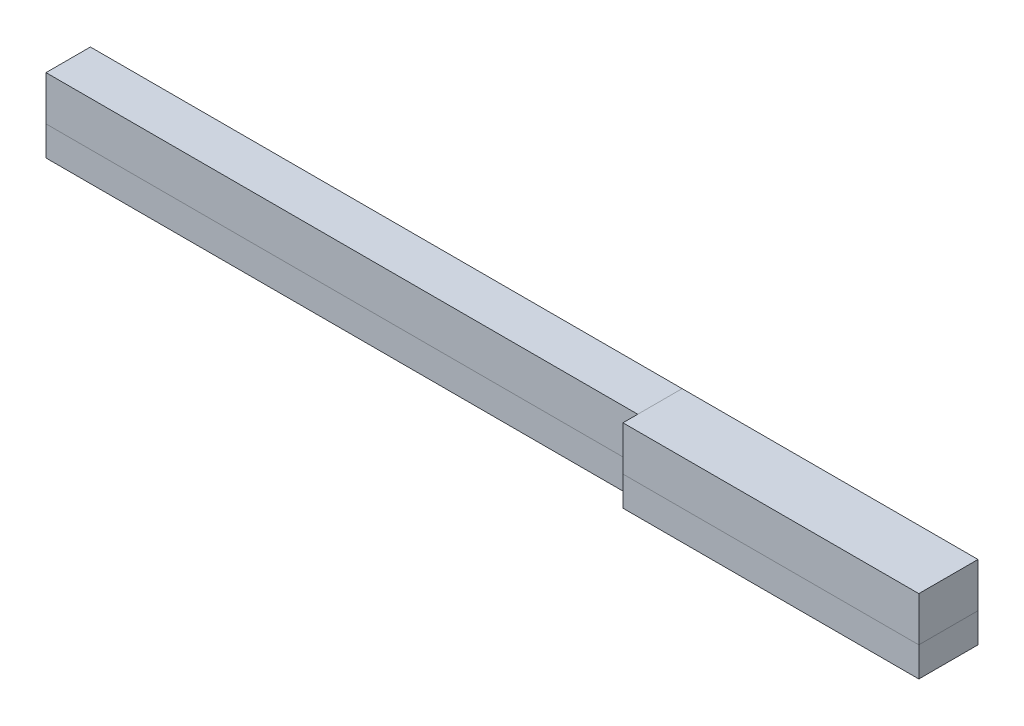
SolidWorks part; units mm, degrees
ref_plane "前视基准面" through (0, 0, 0) normal (0, 0, 1) x (1, 0, 0)
ref_plane "上视基准面" through (0, 0, 0) normal (0, 1, 0) x (1, 0, 0)
ref_plane "右视基准面" through (0, 0, 0) normal (1, 0, 0) x (0, 0, -1)
sketch "草图1" plane through (0, 0, 0) normal (0, 1, 0) x (1, 0, 0)
  line L1 (10, -2) -> (-10, -2)
  line L2 (10, -2) -> (10, 2)
  line L3 (10, 2) -> (-10, 2)
  line L4 (-10, -2) -> (-10, 2)
  line L5 (10, -2) -> (-10, 2) construction
  line L6 (10, 2) -> (-10, -2) construction
  point P0 (0, 0)
  dimension "D1" = 4
  dimension "D2" = 20
extrude "凸台-拉伸1" add sketch "草图1" along normal blind 2
sketch "草图3" plane through (0, 2, 0) normal (0, 1, 0) x (1, 0, 0)
  line L4 (-10, 2) -> (-10, -2)
  line L5 (-10, -2) -> (10, -2)
  line L6 (10, -2) -> (10, 2)
  line L7 (10, 2) -> (-10, 2)
  line L8 (-10, 2) -> (-10, -2)
  line L9 (-10, -2) -> (10, -2)
  line L10 (10, -2) -> (10, 2)
  line L11 (10, 2) -> (-10, 2)
  dimension "D1" = 0
extrude "凸台-拉伸2" add sketch "草图3" along normal blind 3 separate body
sketch "草图4" plane through (0, 0, 0) normal (0, -1, 0) x (1, 0, 0)
  line L0 (10, -2) -> (-10, -2) construction
  line L1 (-10, 1) -> (-50, 1)
  line L2 (-10, 1) -> (-10, -2)
  line L3 (-10, -2) -> (-50, -2)
  line L4 (-50, 1) -> (-50, -2)
  line L5 (-10, -2) -> (-10, 2) construction
  dimension "D1" = 40
  dimension "D2" = 3
extrude "凸台-拉伸3" add sketch "草图4" against normal blind 2 separate body
sketch "草图5" plane through (0, 2, 0) normal (0, 1, 0) x (1, 0, 0)
  line L0 (-10, -1) -> (-50, -1) construction
  line L1 (-50, 2) -> (-10, 2)
  line L2 (-50, 2) -> (-50, -1)
  line L3 (-50, -1) -> (-10, -1)
  line L4 (-10, 2) -> (-10, -1)
  line L5 (-10, 2) -> (-10, -2) construction
extrude "凸台-拉伸4" add sketch "草图5" along normal blind 3 separate body
